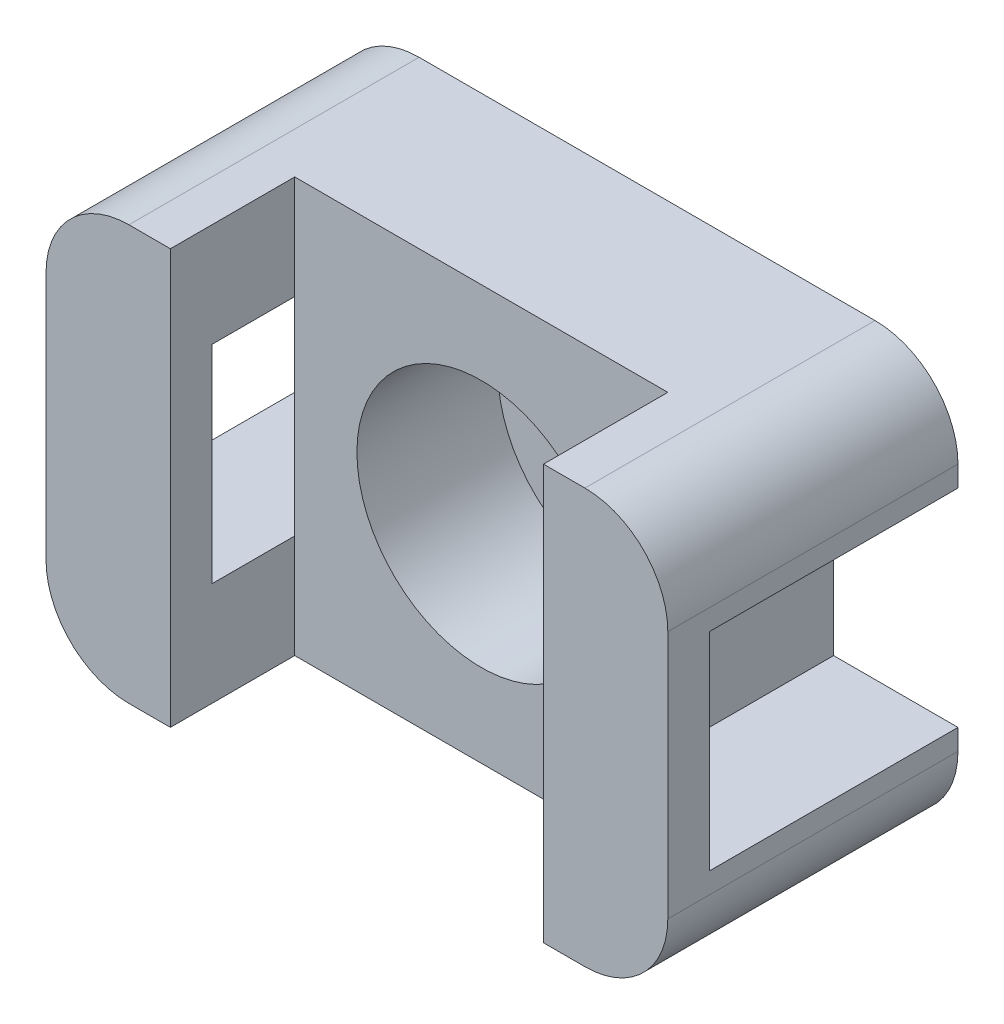
SolidWorks part; units mm, degrees
ref_plane "Front Plane" through (0, 0, 0) normal (0, 0, 1) x (1, 0, 0)
ref_plane "Top Plane" through (0, 0, 0) normal (0, 1, 0) x (1, 0, 0)
ref_plane "Right Plane" through (0, 0, 0) normal (1, 0, 0) x (0, 0, -1)
sketch "Sketch1" plane through (0, 0, 0) normal (0, 0, 1) x (1, 0, 0)
  line L1 (-7.5, -5) -> (7.5, -5)
  line L2 (-7.5, -5) -> (-7.5, 5)
  line L3 (-7.5, 5) -> (7.5, 5)
  line L4 (7.5, -5) -> (7.5, 5)
  line L5 (-7.5, -5) -> (7.5, 5) construction
  line L6 (-7.5, 5) -> (7.5, -5) construction
  point P0 (0, 0)
  dimension "D1" = 15
  dimension "D2" = 10
extrude "Boss-Extrude1" add sketch "Sketch1" along normal blind 7
sketch "Sketch2" plane through (0, 0, 7) normal (0, 0, 1) x (1, 0, 0)
  line L1 (-4.5, -7.8837) -> (4.5, -7.8837)
  line L2 (-4.5, -7.8837) -> (-4.5, 7.8837)
  line L3 (-4.5, 7.8837) -> (4.5, 7.8837)
  line L4 (4.5, -7.8837) -> (4.5, 7.8837)
  line L5 (-4.5, -7.8837) -> (4.5, 7.8837) construction
  line L6 (-4.5, 7.8837) -> (4.5, -7.8837) construction
  point P0 (0, 0)
  dimension "D1" = 9
extrude "Cut-Extrude1" cut sketch "Sketch2" against normal blind 3
sketch "Sketch4" plane through (0, 0, 0) normal (0, 0, -1) x (-1, 0, 0)
  line L0 (-7.5, -5) -> (-7.5, 5) construction
  line L1 (-10.5, -2.5) -> (-4.5, -2.5)
  line L2 (-10.5, -2.5) -> (-10.5, 2.5)
  line L3 (-10.5, 2.5) -> (-4.5, 2.5)
  line L4 (-4.5, -2.5) -> (-4.5, 2.5)
  line L5 (-10.5, -2.5) -> (-4.5, 2.5) construction
  line L6 (-10.5, 2.5) -> (-4.5, -2.5) construction
  line L7 (7.5, 5) -> (7.5, -5) construction
  line L8 (10.5, -2.5) -> (4.5, -2.5)
  line L9 (10.5, -2.5) -> (10.5, 2.5)
  line L10 (10.5, 2.5) -> (4.5, 2.5)
  line L11 (4.5, -2.5) -> (4.5, 2.5)
  line L12 (10.5, -2.5) -> (4.5, 2.5) construction
  line L13 (10.5, 2.5) -> (4.5, -2.5) construction
  point P0 (-7.5, 0)
  point P7 (7.5, 0)
  dimension "D1" = 5
  dimension "D2" = 9
extrude "Cut-Extrude3" cut sketch "Sketch4" against normal blind 6
hole_wizard "Hole size per socket head cap screw type 1" positions "Sketch6" profile "Sketch5" counterbore size "M3" standard "Gb" end condition through all
sketch "Sketch6" plane through (0, 0, 4) normal (0, 0, 1) x (1, 0, 0)
  point P0 (0, 0)
sketch "Sketch5" plane through (0, 0, 4) normal (1, 0, 0) x (0, -1, 0)
  line L0 (0, 0) -> (0, 4)
  line L1 (0, 4) -> (1.7, 4)
  line L3 (1.7, 4) -> (1.7, 3.4)
  line L4 (1.7, 3.4) -> (3, 3.4)
  line L5 (3, 3.4) -> (3, 0)
  line L7 (3, 0) -> (0, 0)
  line L11 (0, -6.35) -> (0, 107.95) construction
  dimension "通孔孔直径" = 3.4
  dimension "通孔孔深度" = 4
  dimension "柱形沉头孔直径" = 6
  dimension "柱形沉头孔深度" = 3.4
fillet "Fillet1" radius 2 4 edges at (-7.5, 5, 3.5) (-7.5, -5, 3.5) (7.5, 5, 3.5) (7.5, -5, 3.5)
